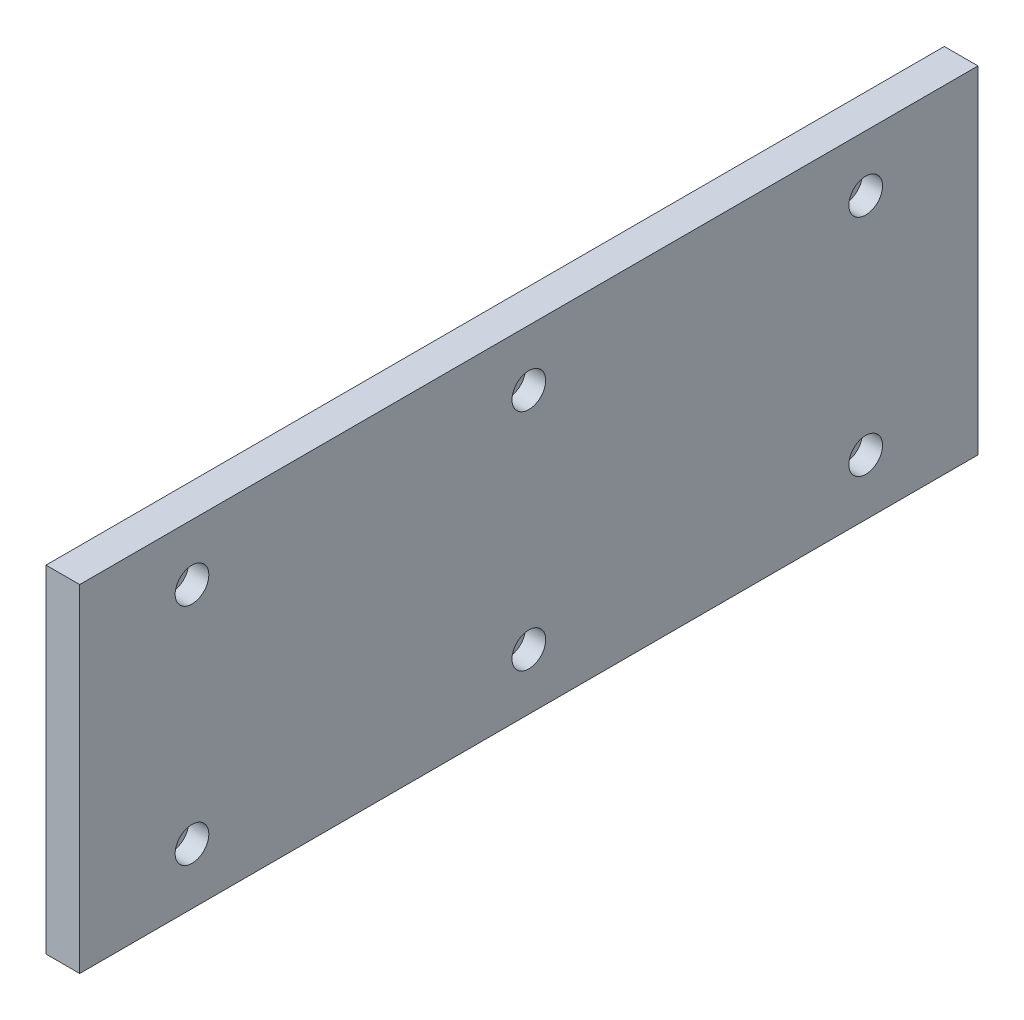
from build123d import *

# Parameters (mm, degrees)
SKETCH_1_W                = 400
SKETCH_1_H                = 150
EXTRUDE_1_DEPTH           = 15
HOLE_WIZARD_1_D           = 9
HOLE_WIZARD_1_CBORE_D     = 15
HOLE_WIZARD_1_CBORE_DEPTH = 9


with BuildPart() as part:
    # 草图1 → 凸台-拉伸1 (new body)
    with BuildSketch(Plane(origin=(0, 0, 0), x_dir=(0, 0, -1), z_dir=(1, 0, 0))):
        Rectangle(SKETCH_1_W, SKETCH_1_H)
    extrude(amount=EXTRUDE_1_DEPTH)

    # 打孔尺寸(%根据)内六角圆柱头螺钉的类型1 (through all)
    with Locations(Plane(origin=(15, 0, 0), x_dir=(0, 0, -1), z_dir=(1, 0, 0))):
        with Locations((-150, 50), (0, 50), (150, 50), (-150, -50), (0, -50), (150, -50)):
            CounterBoreHole(HOLE_WIZARD_1_D / 2, HOLE_WIZARD_1_CBORE_D / 2, HOLE_WIZARD_1_CBORE_DEPTH)


solid = part.part
